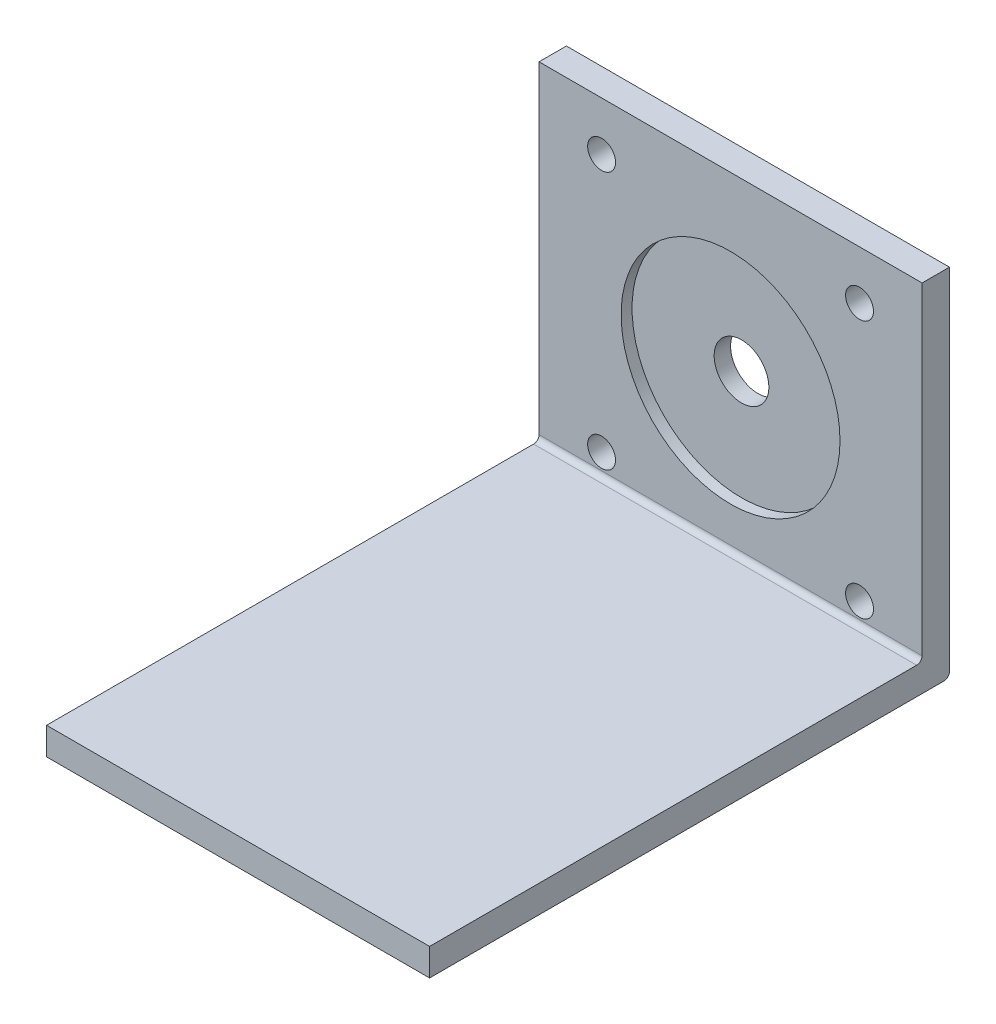
from build123d import *

# Parameters (mm, degrees)
SKETCH_1_W               = 70
SKETCH_1_H               = 65
EXTRUDE_1_DEPTH          = 5
CUT_EXTRUDE_2_DEPTH      = 49.023431781
CUT_EXTRUDE_2_DEPTH_BACK = 49.023431781
SKETCH_3_R               = 2.55
SKETCH_4_W               = 70
SKETCH_4_H               = 5
EXTRUDE_2_DEPTH          = 90
FILLET_1_R               = 1
FILLET_2_R               = 1
CUT_EXTRUDE_START        = -5
SKETCH_5_R               = 20
CUT_EXTRUDE_3_DEPTH      = 2
CUT_EXTRUDE_4_DEPTH      = 104.659297702
CUT_EXTRUDE_4_DEPTH_BACK = 104.659297702
SKETCH_6_R               = 5


with BuildPart() as part:
    # 草图1 → 凸台-拉伸1 (new body)
    with BuildSketch(Plane.XY):
        Rectangle(SKETCH_1_W, SKETCH_1_H)
    extrude(amount=EXTRUDE_1_DEPTH)

    # 草图3 → 切除-拉伸2 (cut, two sides: drawn at the far end of the back side and taken through both)
    with BuildSketch(Plane.XY.offset(5).offset(-CUT_EXTRUDE_2_DEPTH_BACK)):
        with Locations((-23.57, 23.57)):
            Circle(SKETCH_3_R)
        with Locations((23.57, 23.57)):
            Circle(SKETCH_3_R)
        with Locations((23.57, -23.57)):
            Circle(SKETCH_3_R)
        with Locations((-23.57, -23.57)):
            Circle(SKETCH_3_R)
    extrude(amount=CUT_EXTRUDE_2_DEPTH + CUT_EXTRUDE_2_DEPTH_BACK, mode=Mode.SUBTRACT)

    # 草图4 → 凸台-拉伸2 (add)
    with BuildSketch(Plane.XY.offset(5)):
        with Locations((0, -30)):
            Rectangle(SKETCH_4_W, SKETCH_4_H)
    extrude(amount=EXTRUDE_2_DEPTH)

    # 圆角1
    fillet_1_edges = [part.edges().sort_by_distance(p)[0] for p in [
        (0, -27.5, 5),
    ]]
    fillet(fillet_1_edges, radius=FILLET_1_R)

    # 圆角2
    fillet_2_edges = [part.edges().sort_by_distance(p)[0] for p in [
        (0, -32.5, 0),
    ]]
    fillet(fillet_2_edges, radius=FILLET_2_R)

    # 草图5 → 切除-拉伸3 (cut)
    with BuildSketch(Plane(origin=(0, 0, 0), x_dir=(-1, 0, 0), z_dir=(0, 0, -1)).offset(CUT_EXTRUDE_START)):
        with Locations(Location((0, 0, 0), (0, 0, 180))):
            Circle(SKETCH_5_R)
    extrude(amount=CUT_EXTRUDE_3_DEPTH, mode=Mode.SUBTRACT)

    # 草图6 → 切除-拉伸4 (cut, two sides: drawn at the far end of the back side and taken through both)
    with BuildSketch(Plane.XY.offset(3).offset(-CUT_EXTRUDE_4_DEPTH_BACK)):
        Circle(SKETCH_6_R)
    extrude(amount=CUT_EXTRUDE_4_DEPTH + CUT_EXTRUDE_4_DEPTH_BACK, mode=Mode.SUBTRACT)


solid = part.part
